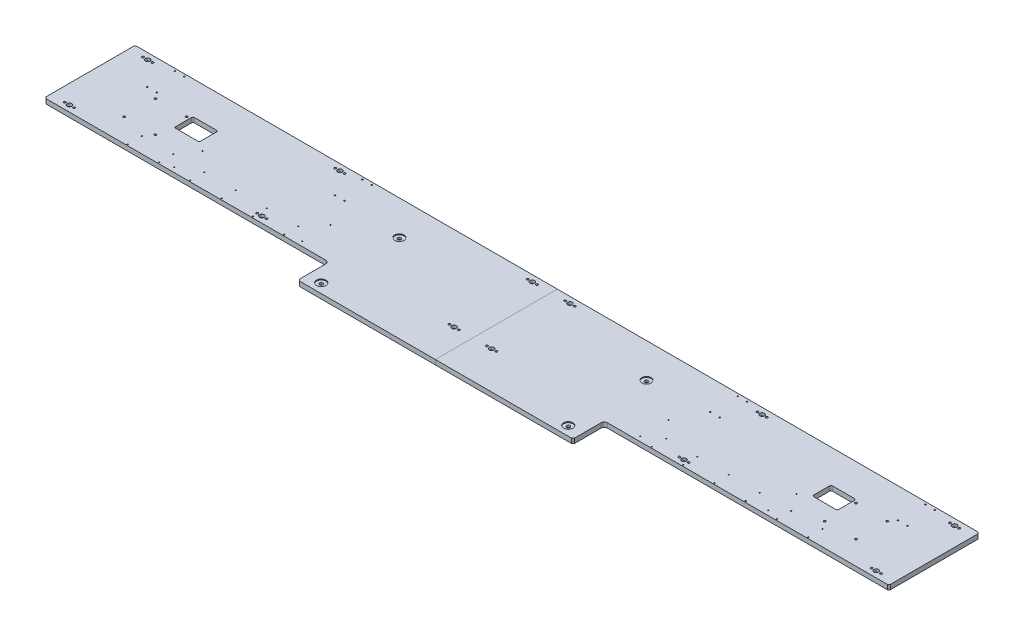
SolidWorks part; units mm, degrees
material "45#"
ref_plane "前基準面" through (0, 0, 0) normal (0, 0, 1) x (1, 0, 0)
ref_plane "上基準面" through (0, 0, 0) normal (0, 1, 0) x (1, 0, 0)
ref_plane "右基準面" through (0, 0, 0) normal (1, 0, 0) x (0, 0, -1)
sketch "草图1" plane through (0, 0, 0) normal (0, 1, 0) x (1, 0, 0)
  line L1 (-1350, 145) -> (1350, 145)
  line L2 (-1350, 145) -> (-1350, -145)
  line L3 (-1350, -145) -> (1350, -145)
  line L4 (1350, 145) -> (1350, -145)
  line L5 (-1350, 145) -> (1350, -145) construction
  line L6 (-1350, -145) -> (1350, 145) construction
  point P0 (0, 0)
  dimension "D1" = 2700
  dimension "D2" = 290
extrude "凸台-拉伸1" add sketch "草图1" along normal blind 20
sketch "草图18" plane through (0, 20, 0) normal (0, 1, 0) x (1, 0, 0)
  line L0 (-1350, -145) -> (1350, -145) construction
  line L1 (-440, -145) -> (440, -145)
  line L2 (-440, -145) -> (-440, -245)
  line L3 (-440, -245) -> (440, -245)
  line L4 (440, -145) -> (440, -245)
  line L5 (0, 0) -> (0, -145) construction
  dimension "D1" = 880
  dimension "D2" = 100
extrude "凸台-拉伸2" add sketch "草图18" against normal up to surface (20 mm away) up to face at (0, 0, 0)
chamfer "倒角1" distance 5 angle 45 6 edges at (1350, 10, -145) (1350, 10, 145) (-1350, 10, -145) (-1350, 10, 145) (440, 10, 245) (-440, 10, 245)
hole_wizard "打孔尺寸(%根据)内六角圆柱头螺钉的类型1" positions "草图2" profile "草图3" counterbore size "M8" standard "GB" end condition through all
sketch "草图2" plane through (0, 20, 0) normal (0, 1, 0) x (1, 0, 0)
  line L0 (-1828.9103, 0) -> (0, 0) construction
  line L1 (0, 0) -> (0, -828.4807) construction
  line L3 (-1345, -145) -> (-440, -145) construction
  line L4 (-1350, 140) -> (-1350, -140) construction
  point P0 (-1290, -125)
  point P11 (-675, -125)
  point P12 (-60, -125)
  point P15 (-675, 125)
  point P16 (-60, 125)
  point P19 (-1290, 125)
  point P32 (1290, 125)
  point P33 (60, 125)
  point P34 (675, 125)
  point P35 (60, -125)
  point P36 (675, -125)
  point P37 (1290, -125)
  dimension "D1" = 3
  dimension "D3" = 615
  dimension "D4" = 20
  dimension "D5" = 60
  dimension "D2" = 2
sketch "草图3" plane through (-1290, 20, 125) normal (1, 0, 0) x (0, 0, 1)
  line L0 (0, 0) -> (0, 20)
  line L1 (0, 20) -> (4.5, 20)
  line L3 (4.5, 20) -> (4.5, 9)
  line L4 (4.5, 9) -> (7.5, 9)
  line L5 (7.5, 9) -> (7.5, 0)
  line L7 (7.5, 0) -> (0, 0)
  line L11 (0, -6.35) -> (0, 107.95) construction
  dimension "通孔孔直径" = 9
  dimension "通孔孔深度" = 20
  dimension "柱形沉头孔直径" = 15
  dimension "柱形沉头孔深度" = 9
hole_wizard "M5 螺纹孔1" positions "草图5" profile "草图6" tap size "M5" standard "GB"
sketch "草图5" plane through (0, 20, 0) normal (0, 1, 0) x (1, 0, 0)
  line L0 (0, 0) -> (0, 640.7675) construction
  line L2 (1345, 145) -> (-1345, 145) construction
  line L3 (-1350, 140) -> (-1350, -140) construction
  point P0 (-585, 49.25)
  point P2 (-615, 49.25)
  point P4 (-1185, 49.25)
  point P6 (-1215, 49.25)
  point P9 (-585, 136.75)
  point P12 (-615, 136.75)
  point P14 (-1185, 136.75)
  point P16 (-1215, 136.75)
  point P23 (1215, 136.75)
  point P24 (1185, 136.75)
  point P25 (615, 136.75)
  point P26 (585, 136.75)
  point P27 (1215, 49.25)
  point P28 (1185, 49.25)
  point P29 (615, 49.25)
  point P30 (585, 49.25)
sketch "草图6" plane through (-585, 20, -49.25) normal (1, 0, 0) x (0, 0, 1)
  line L0 (0, 0) -> (0, 13.6618)
  line L1 (0, 13.6618) -> (2.1, 12.4)
  line L2 (2.1, 12.4) -> (2.1, 0)
  line L5 (2.1, 0) -> (0, 0)
  line L10 (0, 13.6618) -> (-2.1, 12.4) construction
  line L11 (0, -6.35) -> (0, 107.95) construction
  dimension "螺纹孔钻头直径" = 4.2
  dimension "螺纹孔钻头深度" = 12.4
  dimension "导头角度" = 118
cosmetic thread "孔螺蚊线162" parameters "D1"=10, "D2"=5
cosmetic thread "孔螺蚊线163" parameters "D1"=10, "D2"=5
cosmetic thread "孔螺蚊线164" parameters "D1"=10, "D2"=5
cosmetic thread "孔螺蚊线165" parameters "D1"=10, "D2"=5
cosmetic thread "孔螺蚊线166" parameters "D1"=10, "D2"=5
cosmetic thread "孔螺蚊线167" parameters "D1"=10, "D2"=5
cosmetic thread "孔螺蚊线168" parameters "D1"=10, "D2"=5
cosmetic thread "孔螺蚊线169" parameters "D1"=10, "D2"=5
cosmetic thread "孔螺蚊线170" parameters "D1"=10, "D2"=5
cosmetic thread "孔螺蚊线171" parameters "D1"=10, "D2"=5
cosmetic thread "孔螺蚊线172" parameters "D1"=10, "D2"=5
cosmetic thread "孔螺蚊线173" parameters "D1"=10, "D2"=5
cosmetic thread "孔螺蚊线174" parameters "D1"=10, "D2"=5
cosmetic thread "孔螺蚊线175" parameters "D1"=10, "D2"=5
cosmetic thread "孔螺蚊线176" parameters "D1"=10, "D2"=5
cosmetic thread "孔螺蚊线177" parameters "D1"=10, "D2"=5
hole_wizard "M4 螺纹孔1" positions "草图7" profile "草图8" tap size "M4" standard "ISO"
sketch "草图7" plane through (0, 20, 0) normal (0, 1, 0) x (1, 0, 0)
  line L0 (0, 0) -> (0, -370.8913) construction
  line L1 (1350, -140) -> (1350, 140) construction
  line L3 (1345, 145) -> (-1345, 145) construction
  point P0 (540, -40)
  point P2 (950, -130)
  point P4 (540, -130)
  point P6 (950, -40)
  point P14 (-950, -40)
  point P15 (-540, -130)
  point P16 (-950, -130)
  point P17 (-540, -40)
  dimension "D1" = 410
  dimension "D2" = 400
  dimension "D3" = 185
  dimension "D4" = 90
sketch "草图8" plane through (540, 20, 40) normal (1, 0, 0) x (0, 0, 1)
  line L0 (0, 0) -> (0, 11.0914)
  line L1 (0, 11.0914) -> (1.65, 10.1)
  line L2 (1.65, 10.1) -> (1.65, 0)
  line L5 (1.65, 0) -> (0, 0)
  line L10 (0, 11.0914) -> (-1.65, 10.1) construction
  line L11 (0, -6.35) -> (0, 107.95) construction
  dimension "螺纹孔钻头直径" = 3.3
  dimension "螺纹孔钻头深度" = 10.1
  dimension "导头角度" = 118
cosmetic thread "孔螺蚊线178" parameters "D1"=8, "D2"=4
cosmetic thread "孔螺蚊线179" parameters "D1"=8, "D2"=4
cosmetic thread "孔螺蚊线180" parameters "D1"=8, "D2"=4
cosmetic thread "孔螺蚊线181" parameters "D1"=8, "D2"=4
cosmetic thread "孔螺蚊线182" parameters "D1"=8, "D2"=4
cosmetic thread "孔螺蚊线183" parameters "D1"=8, "D2"=4
cosmetic thread "孔螺蚊线184" parameters "D1"=8, "D2"=4
cosmetic thread "孔螺蚊线185" parameters "D1"=8, "D2"=4
hole_wizard "M8 螺纹孔1" positions "草图9" profile "草图10" tap size "M8" standard "GB" end condition through all
sketch "草图9" plane through (0, 20, 0) normal (0, 1, 0) x (1, 0, 0)
  line L0 (-1305, -125) -> (-1290, -125) construction
  line L1 (-1290, -125) -> (-1275, -125) construction
  line L3 (-690, -125) -> (-675, -125) construction
  line L4 (-675, -125) -> (-660, -125) construction
  line L5 (-75, -125) -> (-60, -125) construction
  line L6 (-60, -125) -> (-45, -125) construction
  line L11 (-690, 125) -> (-675, 125) construction
  line L12 (-675, 125) -> (-660, 125) construction
  line L13 (-75, 125) -> (-60, 125) construction
  line L14 (-60, 125) -> (-45, 125) construction
  line L19 (-1305, 125) -> (-1290, 125) construction
  line L20 (-1290, 125) -> (-1275, 125) construction
  line L21 (0, 0) -> (0, -341.3558) construction
  line L22 (1290, 125) -> (1275, 125) construction
  line L23 (1305, 125) -> (1290, 125) construction
  line L24 (60, 125) -> (45, 125) construction
  line L25 (75, 125) -> (60, 125) construction
  line L26 (675, 125) -> (660, 125) construction
  line L27 (690, 125) -> (675, 125) construction
  line L28 (60, -125) -> (45, -125) construction
  line L29 (75, -125) -> (60, -125) construction
  line L30 (675, -125) -> (660, -125) construction
  line L31 (690, -125) -> (675, -125) construction
  line L32 (1290, -125) -> (1275, -125) construction
  line L33 (1305, -125) -> (1290, -125) construction
  circle A0 centre (-675, -125) radius 4.5 construction
  point P0 (-1305, -125)
  point P2 (-1275, -125)
  point P16 (-690, -125)
  point P17 (-660, -125)
  point P21 (-75, -125)
  point P22 (-45, -125)
  point P36 (-690, 125)
  point P37 (-660, 125)
  point P41 (-75, 125)
  point P42 (-45, 125)
  point P56 (-1305, 125)
  point P57 (-1275, 125)
  point P91 (1275, 125)
  point P92 (1305, 125)
  point P93 (45, 125)
  point P94 (75, 125)
  point P95 (660, 125)
  point P96 (690, 125)
  point P97 (45, -125)
  point P98 (75, -125)
  point P99 (660, -125)
  point P100 (690, -125)
  point P101 (1275, -125)
  point P102 (1305, -125)
  dimension "D1" = 30
  dimension "D2" = 3
  dimension "D3" = 2
sketch "草图10" plane through (-1305, 20, 125) normal (1, 0, 0) x (0, 0, 1)
  line L0 (0, 0) -> (0, 20)
  line L1 (0, 20) -> (3.4, 20)
  line L2 (3.4, 20) -> (3.4, 0)
  line L5 (3.4, 0) -> (0, 0)
  line L11 (0, -6.35) -> (0, 107.95) construction
  dimension "通孔螺纹孔钻头直径" = 6.8
  dimension "通孔螺纹孔钻头深度" = 20
cosmetic thread "孔螺蚊线27"
cosmetic thread "孔螺蚊线133"
cosmetic thread "孔螺蚊线134"
cosmetic thread "孔螺蚊线135"
cosmetic thread "孔螺蚊线136"
cosmetic thread "孔螺蚊线137"
cosmetic thread "孔螺蚊线138"
cosmetic thread "孔螺蚊线139"
cosmetic thread "孔螺蚊线140"
cosmetic thread "孔螺蚊线141"
cosmetic thread "孔螺蚊线142"
cosmetic thread "孔螺蚊线143"
cosmetic thread "孔螺蚊线144"
cosmetic thread "孔螺蚊线145"
cosmetic thread "孔螺蚊线146"
cosmetic thread "孔螺蚊线147"
cosmetic thread "孔螺蚊线148"
cosmetic thread "孔螺蚊线149"
cosmetic thread "孔螺蚊线150"
cosmetic thread "孔螺蚊线151"
cosmetic thread "孔螺蚊线152"
cosmetic thread "孔螺蚊线153"
cosmetic thread "孔螺蚊线154"
cosmetic thread "孔螺蚊线155"
sketch "草图11" plane through (0, 20, 0) normal (0, 1, 0) x (1, 0, 0)
  line L0 (0, 0) -> (0, -269.0218) construction
  line L1 (-1055, 40) -> (-985, 40)
  line L2 (-1060, 35) -> (-1060, -15)
  line L3 (-1055, -20) -> (-985, -20)
  line L4 (-980, 35) -> (-980, -15)
  line L5 (980, 35) -> (980, -15)
  line L6 (1055, -20) -> (985, -20)
  line L7 (1060, 35) -> (1060, -15)
  line L8 (1055, 40) -> (985, 40)
  line L9 (-1345, -145) -> (-440, -145) construction
  arc A0 (-1055, 40) -> (-1060, 35) centre (-1055, 35) ccw
  arc A1 (-985, 40) -> (-980, 35) centre (-985, 35) cw
  arc A2 (-985, -20) -> (-980, -15) centre (-985, -15) ccw
  arc A3 (-1060, -15) -> (-1055, -20) centre (-1055, -15) ccw
  arc A4 (1060, -15) -> (1055, -20) centre (1055, -15) cw
  arc A5 (985, -20) -> (980, -15) centre (985, -15) cw
  arc A6 (985, 40) -> (980, 35) centre (985, 35) ccw
  arc A7 (1055, 40) -> (1060, 35) centre (1055, 35) cw
  circle A8 centre (-950, -130) radius 1.65 construction
  dimension "D1" = 5
  dimension "D2" = 30
  dimension "D3" = 60
  dimension "D4" = 125
  dimension "D5" = 80
extrude "切除-拉伸1" cut sketch "草图11" against normal up to surface (20 mm away) up to face at (-1305, 0, 128.4)
hole_wizard "打孔尺寸(%根据)内六角圆柱头螺钉的类型3" positions "草图12" profile "草图13" counterbore size "M10" standard "GB" end condition through all
sketch "草图12" plane through (0, 0, 0) normal (0, -1, 0) x (-1, 0, 0)
  line L0 (0, 0) -> (0, -515.6294) construction
  line L2 (435, -245) -> (-435, -245) construction
  point P0 (395, -215)
  point P2 (395, 35)
  point P8 (-395, 35)
  point P9 (-395, -215)
  dimension "D1" = 250
  dimension "D2" = 30
  dimension "D3" = 790
sketch "草图13" plane through (-395, 0, 215) normal (1, 0, 0) x (0, 0, -1)
  line L0 (0, 0) -> (0, 20)
  line L1 (0, 20) -> (5.5, 20)
  line L3 (5.5, 20) -> (5.5, 11)
  line L4 (5.5, 11) -> (9, 11)
  line L5 (9, 11) -> (9, 0)
  line L7 (9, 0) -> (0, 0)
  line L11 (0, -6.35) -> (0, 107.95) construction
  dimension "通孔孔直径" = 11
  dimension "通孔孔深度" = 20
  dimension "柱形沉头孔直径" = 18
  dimension "柱形沉头孔深度" = 11
fillet "圆角1" radius 10 2 edges at (-440, 10, 145) (440, 10, 145)
hole_wizard "M8 螺纹孔2" positions "草图19" profile "草图20" tap size "M8" standard "GB" end condition through all
sketch "草图19" plane through (0, 20, 0) normal (0, 1, 0) x (1, 0, 0)
  line L0 (0, 0) -> (0, 368.4409) construction
  line L3 (450, -145) -> (1345, -145) construction
  point P0 (1170, 30)
  point P2 (1070, 30)
  point P4 (1070, -70)
  point P6 (1170, -70)
  point P13 (-1170, -70)
  point P14 (-1070, -70)
  point P15 (-1070, 30)
  point P16 (-1170, 30)
  dimension "D1" = 100
  dimension "D2" = 2240
  dimension "D3" = 100
  dimension "D4" = 75
sketch "草图20" plane through (1170, 20, -30) normal (1, 0, 0) x (0, 0, 1)
  line L0 (0, 0) -> (0, 20)
  line L1 (0, 20) -> (3.4, 20)
  line L2 (3.4, 20) -> (3.4, 0)
  line L5 (3.4, 0) -> (0, 0)
  line L11 (0, -6.35) -> (0, 107.95) construction
  dimension "通孔螺纹孔钻头直径" = 6.8
  dimension "通孔螺纹孔钻头深度" = 20
cosmetic thread "孔螺蚊线69" parameters "D2"=8
cosmetic thread "孔螺蚊线70" parameters "D2"=8
cosmetic thread "孔螺蚊线156" parameters "D2"=8
cosmetic thread "孔螺蚊线157" parameters "D2"=8
cosmetic thread "孔螺蚊线158" parameters "D2"=8
cosmetic thread "孔螺蚊线159" parameters "D2"=8
cosmetic thread "孔螺蚊线160" parameters "D2"=8
cosmetic thread "孔螺蚊线161" parameters "D2"=8
sketch "草图21" plane through (0, 20, 0) normal (0, -1, 0) x (1, 0, 0)
  line L0 (0, 0) -> (0, 326.2943) construction
  circle A0 centre (395, 215) radius 15
  circle A1 centre (395, -35) radius 15
  circle A2 centre (-395, -35) radius 15
  circle A3 centre (-395, 215) radius 15
  dimension "D1" = 30
extrude "切除-拉伸2" cut sketch "草图21" along normal blind 3
hole_wizard "M4 螺纹孔2" positions "草图22" profile "草图23" tap size "M4" standard "GB" end condition through all
sketch "草图22" plane through (0, 20, 0) normal (0, 1, 0) x (1, 0, 0)
  line L0 (-1350, 140) -> (-1350, -140) construction
  line L1 (-1345, -145) -> (-450, -145) construction
  line L2 (0, 0) -> (0, -455.7132) construction
  point P0 (-1088, -95.5)
  point P2 (-1088, -140.5)
  point P11 (-988, -95.5)
  point P12 (-988, -140.5)
  point P13 (-888, -95.5)
  point P14 (-888, -140.5)
  point P15 (-788, -95.5)
  point P16 (-788, -140.5)
  point P17 (-688, -95.5)
  point P18 (-688, -140.5)
  point P29 (688, -140.5)
  point P30 (688, -95.5)
  point P31 (788, -140.5)
  point P32 (788, -95.5)
  point P33 (888, -140.5)
  point P34 (888, -95.5)
  point P35 (988, -140.5)
  point P36 (988, -95.5)
  point P37 (1088, -140.5)
  point P38 (1088, -95.5)
  point P39 (-588, -95.5)
  point P40 (-588, -140.5)
  point P41 (588, -140.5)
  point P42 (588, -95.5)
  dimension "D1" = 6
  dimension "D2" = 262
  dimension "D3" = 45
  dimension "D4" = 4.5
  dimension "D5" = 100
sketch "草图23" plane through (-1088, 20, 95.5) normal (1, 0, 0) x (0, 0, 1)
  line L0 (0, 0) -> (0, 20)
  line L1 (0, 20) -> (1.65, 20)
  line L2 (1.65, 20) -> (1.65, 0)
  line L5 (1.65, 0) -> (0, 0)
  line L11 (0, -6.35) -> (0, 107.95) construction
  dimension "通孔螺纹孔钻头直径" = 3.3
  dimension "通孔螺纹孔钻头深度" = 20
cosmetic thread "孔螺蚊线74" [suppressed]
cosmetic thread "孔螺蚊线110"
cosmetic thread "孔螺蚊线111"
cosmetic thread "孔螺蚊线112"
cosmetic thread "孔螺蚊线113"
cosmetic thread "孔螺蚊线114"
cosmetic thread "孔螺蚊线115"
cosmetic thread "孔螺蚊线116"
cosmetic thread "孔螺蚊线117"
cosmetic thread "孔螺蚊线118"
cosmetic thread "孔螺蚊线119"
cosmetic thread "孔螺蚊线120"
cosmetic thread "孔螺蚊线121"
cosmetic thread "孔螺蚊线122"
cosmetic thread "孔螺蚊线123"
cosmetic thread "孔螺蚊线124"
cosmetic thread "孔螺蚊线125"
cosmetic thread "孔螺蚊线126"
cosmetic thread "孔螺蚊线127"
cosmetic thread "孔螺蚊线128"
cosmetic thread "孔螺蚊线129"
cosmetic thread "孔螺蚊线130"
cosmetic thread "孔螺蚊线131"
cosmetic thread "孔螺蚊线132"
sketch "草图24" plane through (0, 20, 0) normal (0, 1, 0) x (1, 0, 0)
  line L0 (0, 145) -> (0, -245)
  line L1 (1345, 145) -> (-1345, 145) construction
  line L2 (-435, -245) -> (435, -245) construction
split line "分割线1"
sketch "草图25" plane through (0, 0, 0) normal (0, -1, 0) x (1, 0, 0)
  line L1 (-1617.2524, 642.571) -> (1607.0847, 642.571)
  line L2 (-1617.2524, 642.571) -> (-1617.2524, -580.3692)
  line L3 (-1617.2524, -580.3692) -> (1607.0847, -580.3692)
  line L4 (1607.0847, 642.571) -> (1607.0847, -580.3692)
extrude "切除-拉伸3" cut sketch "草图25" against normal blind 5
equation "\"D4@草图5\"=\"D2@草图5\""
